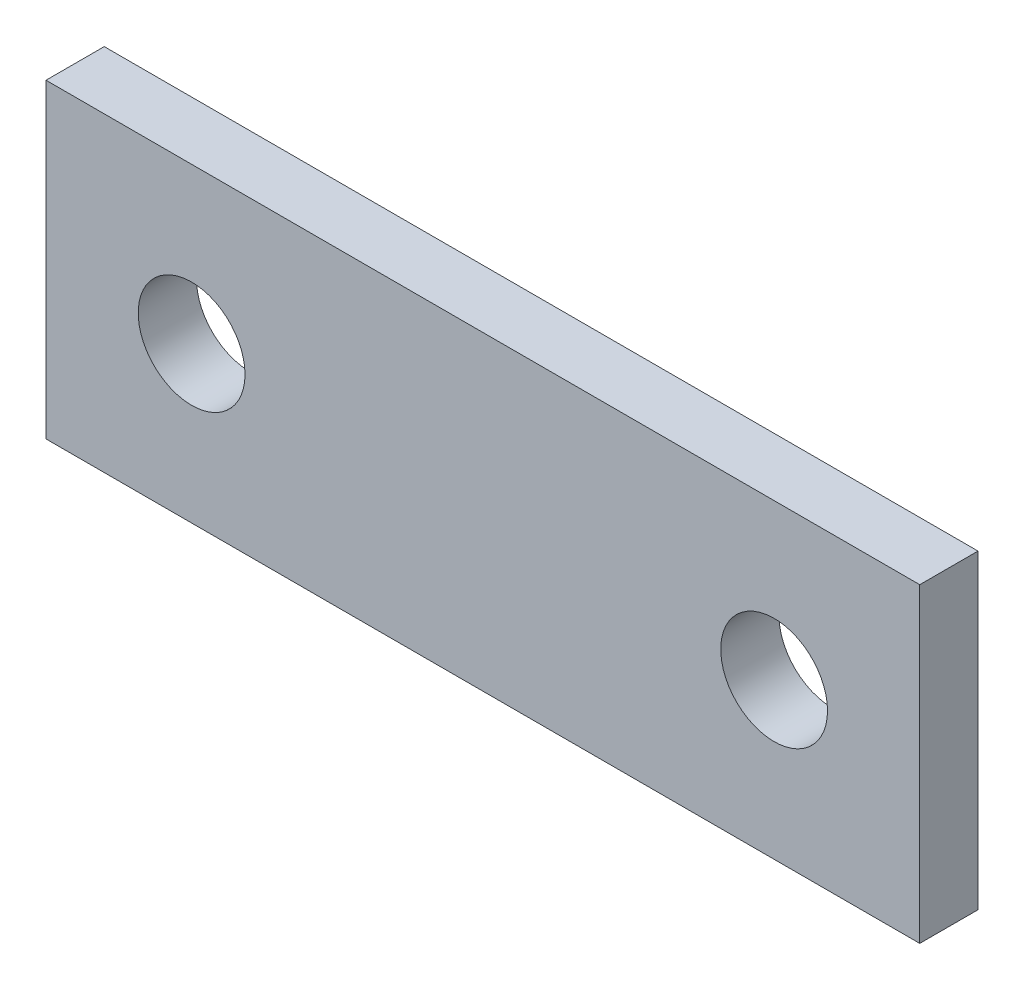
from build123d import *

# Parameters (mm, degrees)
SKETCH1_W           = 90
SKETCH1_H           = 32
BOSS_EXTRUDE1_DEPTH = 6
SKETCH2_R           = 5.5
CUT_EXTRUDE1_DEPTH  = 6
LPATTERN1_COUNT     = 2
LPATTERN1_PITCH     = 60


with BuildPart() as part:
    # Sketch1 → Boss-Extrude1 (new body)
    with BuildSketch(Plane.XY):
        with Locations((45, -16)):
            Rectangle(SKETCH1_W, SKETCH1_H)
    extrude(amount=BOSS_EXTRUDE1_DEPTH)

    # Sketch2 → Cut-Extrude1 (cut)
    with BuildSketch(Plane.XY.offset(6)):
        with Locations((15, -16)):
            Circle(SKETCH2_R)
    cut_extrude1 = extrude(amount=-CUT_EXTRUDE1_DEPTH, mode=Mode.SUBTRACT)

    # LPattern1: Cut-Extrude1 ×2
    with Locations(*[(i * LPATTERN1_PITCH, 0, 0) for i in range(1, LPATTERN1_COUNT)]):
        add(cut_extrude1, mode=Mode.SUBTRACT)


solid = part.part
